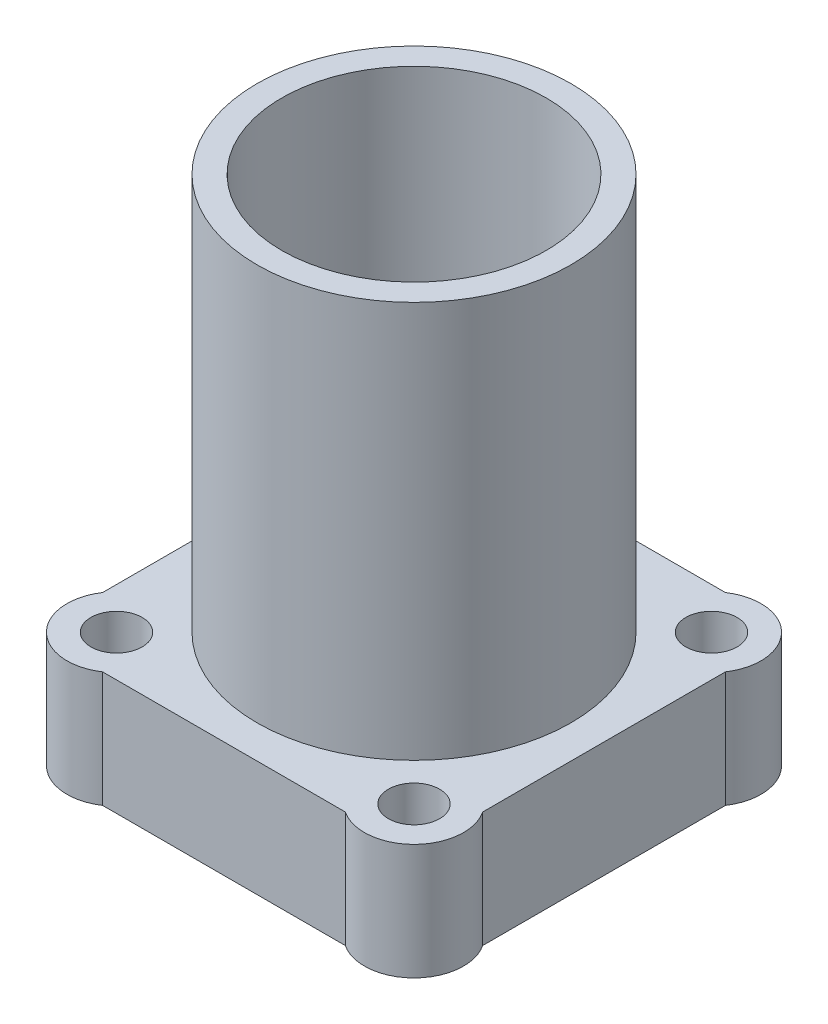
from build123d import *

# Parameters (mm, degrees)
SKETCH_1_R      = 7
SKETCH_1_R_2    = 3
SKETCH_1_R_3    = 1.55
EXTRUDE_1_DEPTH = 7
SKETCH_2_R      = 9.5
SKETCH_2_R_2    = 8
EXTRUDE_2_DEPTH = 24


with BuildPart() as part:
    # 草图1 → 凸台-拉伸1 (new body)
    # profile 1 of 5: a face of its own
    with BuildSketch(Plane(origin=(0, 0, 0), x_dir=(1, 0, 0), z_dir=(0, 1, 0))):
        with BuildLine():
            Line((7.341687605, 11.5), (-7.341687605, 11.5))
            ThreePointArc((-7.341687605, 11.5), (-6.356617963, 10.418637165), (-6, 9))
            ThreePointArc((-6, 9), (-8.133974596, 6.127718677), (-11.5, 7.341687605))
            Line((-11.5, 7.341687605), (-11.5, -7.341687605))
            ThreePointArc((-11.5, -7.341687605), (-8.133974596, -6.127718677), (-6, -9))
            ThreePointArc((-6, -9), (-6.356617963, -10.418637165), (-7.341687605, -11.5))
            Line((-7.341687605, -11.5), (7.341687605, -11.5))
            ThreePointArc((7.341687605, -11.5), (6.878679656, -6.878679656), (11.5, -7.341687605))
            Line((11.5, -7.341687605), (11.5, 7.341687605))
            ThreePointArc((11.5, 7.341687605), (6.878679656, 6.878679656), (7.341687605, 11.5))
        make_face()
        with Locations(Location((0, 0, 0), (0, 0, 270))):
            Circle(SKETCH_1_R, mode=Mode.SUBTRACT)
    # profile 2 of 5: a face of its own
    with BuildSketch(Plane(origin=(0, 0, 0), x_dir=(1, 0, 0), z_dir=(0, 1, 0))):
        with Locations((-9, -9)):
            Circle(SKETCH_1_R_2)
        with Locations(Location((-9, -9, 0), (0, 0, 270))):
            Circle(SKETCH_1_R_3, mode=Mode.SUBTRACT)
    # profile 3 of 5: a face of its own
    with BuildSketch(Plane(origin=(0, 0, 0), x_dir=(1, 0, 0), z_dir=(0, 1, 0))):
        with Locations((9, -9)):
            Circle(SKETCH_1_R_2)
        with Locations(Location((9, -9, 0), (0, 0, 270))):
            Circle(SKETCH_1_R_3, mode=Mode.SUBTRACT)
    # profile 4 of 5: a face of its own
    with BuildSketch(Plane(origin=(0, 0, 0), x_dir=(1, 0, 0), z_dir=(0, 1, 0))):
        with Locations((9, 9)):
            Circle(SKETCH_1_R_2)
        with Locations(Location((9, 9, 0), (0, 0, 270))):
            Circle(SKETCH_1_R_3, mode=Mode.SUBTRACT)
    # profile 5 of 5: a face of its own
    with BuildSketch(Plane(origin=(0, 0, 0), x_dir=(1, 0, 0), z_dir=(0, 1, 0))):
        with Locations((-9, 9)):
            Circle(SKETCH_1_R_2)
        with Locations(Location((-9, 9, 0), (0, 0, 270))):
            Circle(SKETCH_1_R_3, mode=Mode.SUBTRACT)
    extrude(amount=EXTRUDE_1_DEPTH)

    # 草图2 → 凸台-拉伸2 (add)
    with BuildSketch(Plane(origin=(0, 7, 0), x_dir=(1, 0, 0), z_dir=(0, 1, 0))):
        with Locations(Location((0, 0, 0), (0, 0, 270))):
            Circle(SKETCH_2_R)
        with Locations(Location((0, 0, 0), (0, 0, 270))):
            Circle(SKETCH_2_R_2, mode=Mode.SUBTRACT)
    extrude(amount=EXTRUDE_2_DEPTH)


solid = part.part
